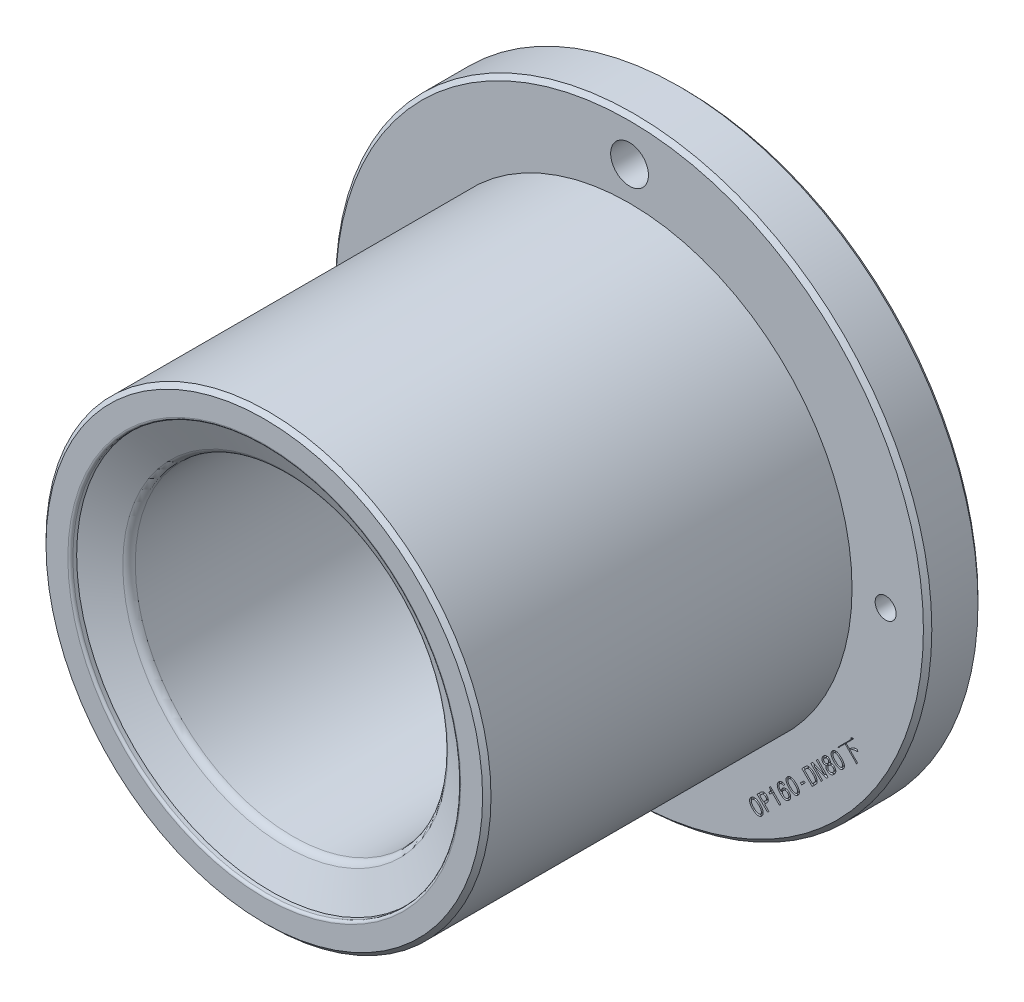
SolidWorks part; units mm, degrees
material "Cr12MoV"
ref_plane "Front/Back" through (0, 0, 0) normal (0, 0, 1) x (1, 0, 0)
ref_plane "Top/Bottom" through (0, 0, 0) normal (0, 1, 0) x (1, 0, 0)
ref_plane "Right/Left" through (0, 0, 0) normal (1, 0, 0) x (0, 0, -1)
sketch "Sketch1" plane through (0, 0, 0) normal (0, 0, 1) x (1, 0, 0)
  circle A0 centre (0, 0) radius 53
  dimension "D1" = 106
extrude "Boss-Extrude1" add sketch "Sketch1" along normal blind 100
sketch "Sketch2" plane through (0, 0, 0) normal (0, 0, -1) x (-1, 0, 0)
  circle A0 centre (0, 0) radius 17.5
  dimension "D1" = 35
extrude "Boss-Extrude2" add sketch "Sketch2" along normal blind 6
sketch "Sketch4" plane through (0, 0, 0) normal (0, 1, 0) x (1, 0, 0)
  line L0 (0, 50.1438) -> (0, -108.1933) construction
  line L1 (46.2, -100) -> (46.2, -98.5)
  line L2 (-53, -100) -> (53, -100) construction
  line L3 (46.2, -98.5) -> (37.55, -94.4664)
  line L4 (37.55, -94.4664) -> (37.55, -15)
  line L5 (37.55, -15) -> (0, -15)
  line L6 (0, -15) -> (0, -100)
  line L7 (0, -100) -> (46.2, -100)
  dimension "D1" = 115
  dimension "D2" = 1.5
  dimension "D3" = 37.55
  dimension "D4" = 46.2
  dimension "D5" = 85
revolve "Cut-Revolve1" cut sketch "Sketch4" angle 360 about L0
fillet "Fillet3" radius 2 1 edges at (-37.55, 0, 94.4664)
chamfer "Chamfer3" distance 1 angle 45 1 edges at (-17.5, 0, -6)
chamfer "Chamfer5" distance 1 angle 45 1 edges at (53, 0, 100)
sketch "Sketch10" plane through (0, 0, 15) normal (0, 0, 1) x (1, 0, 0)
  circle A0 centre (0, 0) radius 4
  dimension "D1" = 8
extrude "Cut-Extrude2" cut sketch "Sketch10" against normal blind 8.5
hole_wizard "M6 Tapped Hole1" positions "Sketch11" profile "Sketch12" tap size "M6" standard "GB" end condition through all
sketch "Sketch11" plane through (0, 0, 6.5) normal (0, 0, 1) x (1, 0, 0)
  point P0 (0, 0)
cosmetic thread "Cosmetic thread 1" parameters "D2"=6
sketch "Sketch12" plane through (0, 0, 6.5) normal (1, 0, 0) x (0, -1, 0)
  line L0 (0, 0) -> (0, 12.5)
  line L1 (0, 12.5) -> (2.5, 12.5)
  line L2 (2.5, 12.5) -> (2.5, 0)
  line L5 (2.5, 0) -> (0, 0)
  line L11 (0, -6.35) -> (0, 107.95) construction
  dimension "通孔螺纹孔钻头直径" = 5
  dimension "通孔螺纹孔钻头深度" = 12.5
sketch "Sketch13" plane through (0, 0, 15) normal (0, 0, 1) x (1, 0, 0)
  circle A0 centre (0, 0) radius 8.75
  dimension "D1" = 17.5
extrude "Cut-Extrude3" cut sketch "Sketch13" against normal blind 5.5
chamfer "Chamfer8" distance 0.5 angle 45 2 edges at (4, 0, 9.5) (8.75, 0, 15)
sketch "Sketch14" plane through (0, 0, 0) normal (0, 0, -1) x (-1, 0, 0)
  circle A0 centre (0, 0) radius 53
  circle A1 centre (0, 0) radius 71
  circle A2 centre (0, 0) radius 53 construction
  dimension "D1" = 142
extrude "Boss-Extrude3" add sketch "Sketch14" against normal blind 13
hole_wizard "M8 Clearance Hole1" positions "Sketch15" profile "Sketch16" hole size "M8" standard "GB" end condition through all
sketch "Sketch15" plane through (0, 0, 13) normal (0, 0, 1) x (1, 0, 0)
  line L0 (0, 71) -> (0, -71) construction
  circle A0 centre (0, 0) radius 71 construction
  circle A1 centre (0, 0) radius 61
  point P0 (0, 61)
  point P2 (0, -61)
  dimension "D1" = 122
sketch "Sketch16" plane through (0, 61, 13) normal (1, 0, 0) x (0, -1, 0)
  line L0 (0, 0) -> (0, 19)
  line L1 (0, 19) -> (4.5, 19)
  line L2 (4.5, 19) -> (4.5, 0)
  line L5 (4.5, 0) -> (0, 0)
  line L11 (0, -6.35) -> (0, 107.95) construction
  dimension "通孔孔直径" = 9
  dimension "通孔孔深度" = 19
chamfer "Chamfer9" distance 1 angle 45 2 edges at (-71, 0, 13) (-71, 0, 0)
fillet "Fillet4" radius 0.6 1 edges at (-46.2, 0, 100)
fillet "Fillet5" radius 8 1 edges at (-37.55, 0, 15)
hole_wizard "M6 Tapped Hole2" positions "Sketch17" profile "Sketch18" tap size "M6" standard "GB"
sketch "Sketch17" plane through (0, 0, 13) normal (0, 0, 1) x (1, 0, 0)
  circle A0 centre (0, 0) radius 61
  point P0 (-61, 0)
  point P9 (61, 0)
sketch "Sketch18" plane through (-61, 0, 13) normal (1, 0, 0) x (0, -1, 0)
  line L0 (0, 0) -> (0, 18.5022)
  line L1 (0, 18.5022) -> (2.5, 17)
  line L2 (2.5, 17) -> (2.5, 0)
  line L5 (2.5, 0) -> (0, 0)
  line L10 (0, 18.5022) -> (-2.5, 17) construction
  line L11 (0, -6.35) -> (0, 107.95) construction
  dimension "螺纹孔钻头直径" = 5
  dimension "螺纹孔钻头深度" = 17
  dimension "导头角度" = 118
cosmetic thread "Cosmetic thread 2" parameters "D1"=12, "D2"=6
cosmetic thread "Cosmetic thread 3" parameters "D1"=12, "D2"=6
sketch "Sketch19" plane through (0, 0, 13) normal (0, 0, 1) x (1, 0, 0)
  line L0 (0, 0) -> (44.5477, -44.5477) construction
  line L1 (0, 0) -> (0, -93.7283) construction
  line L2 (30.4056, -58.6899) -> (58.6899, -30.4056) construction
  text T0 "PF160-DN80下" font "Monospac821 BT" height 3.5
  dimension "D1" = 45
  dimension "D2" = 63
  dimension "D3" = 40
extrude "Cut-Extrude4" cut sketch "Sketch19" against normal blind 0.5
